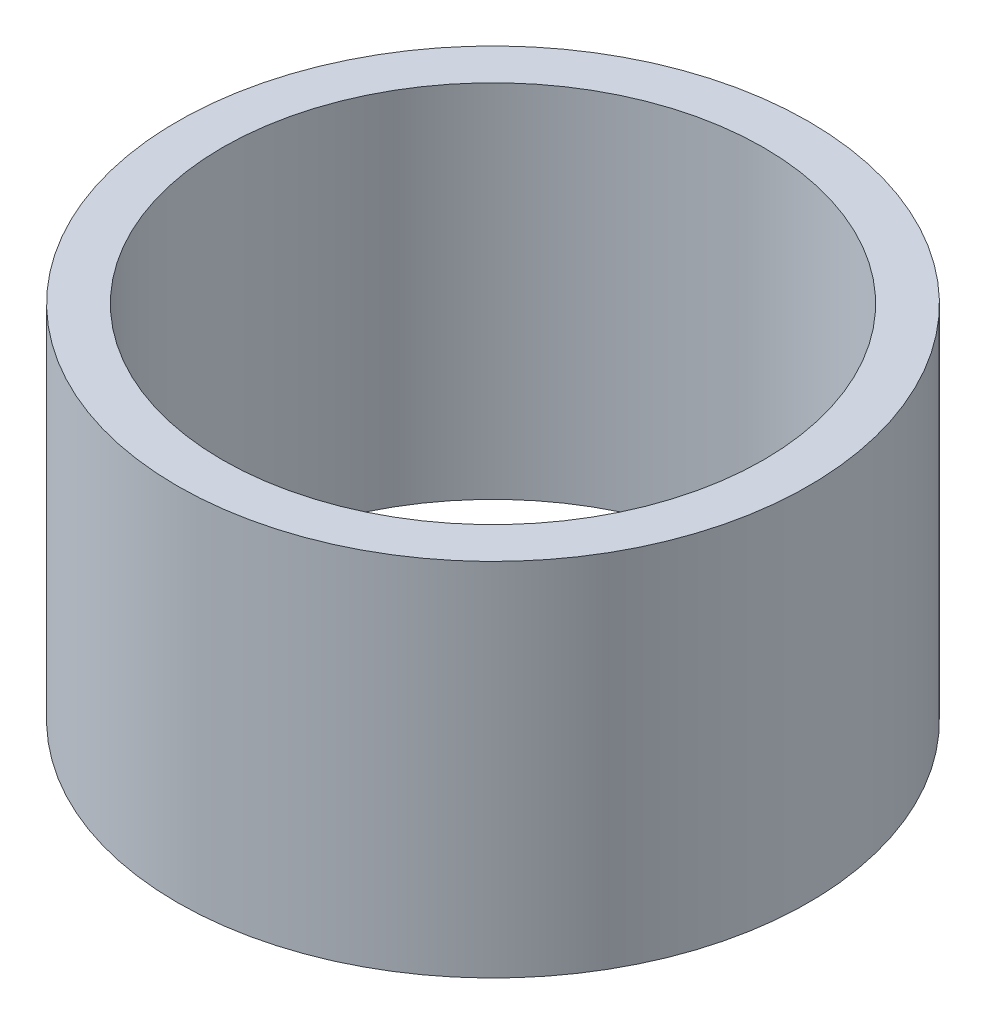
SolidWorks part; units mm, degrees
material "Tin Bearing Bronze"
ref_plane "Front Plane" through (0, 0, 0) normal (0, 0, 1) x (1, 0, 0)
ref_plane "Top Plane" through (0, 0, 0) normal (0, 1, 0) x (1, 0, 0)
ref_plane "Right Plane" through (0, 0, 0) normal (1, 0, 0) x (0, 0, -1)
other "Configuration Table"
sketch "Sketch1" plane through (0, 0, 0) normal (0, 1, 0) x (1, 0, 0)
  circle A0 centre (0, 0) radius 6
  circle A1 centre (0, 0) radius 7
  dimension "D1" = 12
  dimension "D2" = 14
extrude "Boss-Extrude1" add sketch "Sketch1" along normal blind 8
